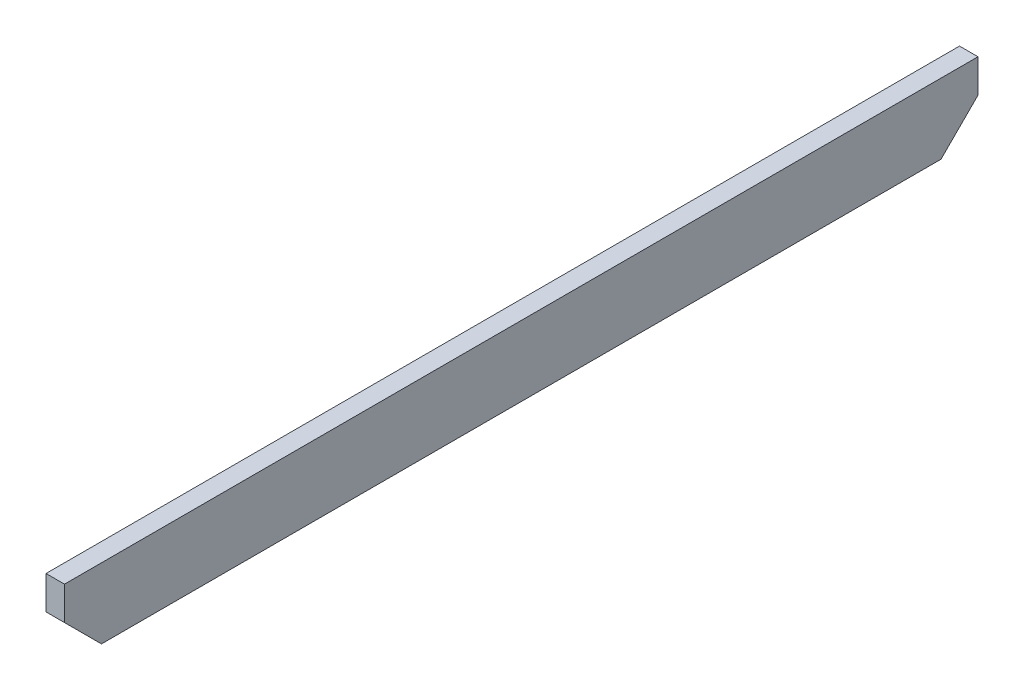
from build123d import *

# Parameters (mm, degrees)
SKETCH_1_W      = 247
SKETCH_1_H      = 19
EXTRUDE_1_DEPTH = 2.5
CHAMFER_1_SIZE  = 10


with BuildPart() as part:
    # 草图1 → 凸台-拉伸1 (new, symmetric)
    with BuildSketch(Plane(origin=(0, 0, 0), x_dir=(0, 0, -1), z_dir=(1, 0, 0))):
        Rectangle(SKETCH_1_W, SKETCH_1_H)
    extrude(amount=EXTRUDE_1_DEPTH, both=True)

    # 倒角1
    chamfer_1_edges = [part.edges().sort_by_distance(p)[0] for p in [
        (0, -9.5, -123.5),
        (0, -9.5, 123.5),
    ]]
    chamfer(chamfer_1_edges, length=CHAMFER_1_SIZE)


solid = part.part
